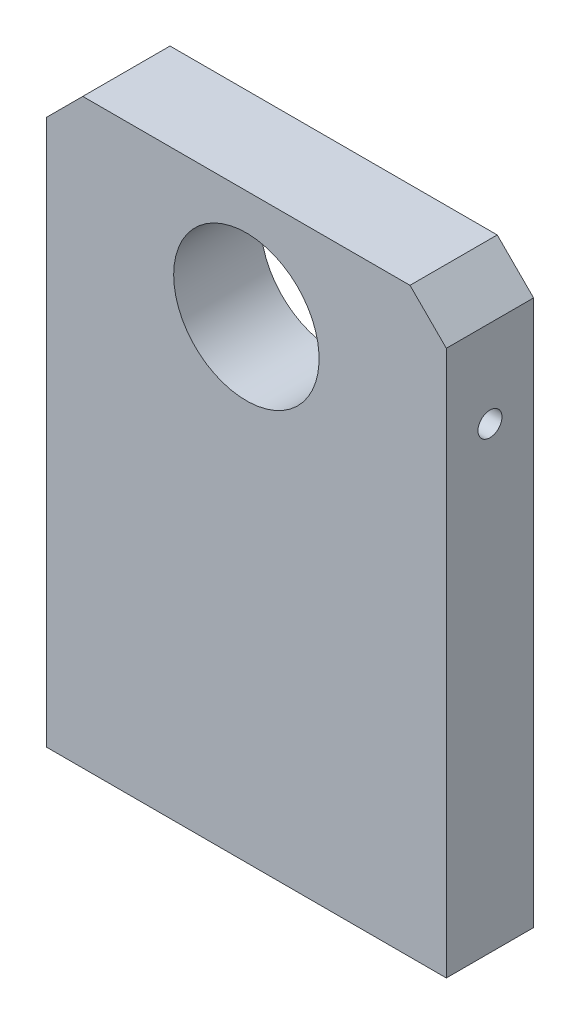
from build123d import *

# Parameters (mm, degrees)
SKETCH_1_W              = 55
SKETCH_1_H              = 80
EXTRUDE_1_DEPTH         = 12
CUT_EXTRUDE_4_REACH     = 52.002
SKETCH_5_R              = 10
CHAMFER_1_SIZE          = 5
HOLE_WIZARD_M4_1_REACH  = 85.845
HOLE_WIZARD_M4_1_BORE_R = 1.65


with BuildPart() as part:
    # 草图1 → 凸台-拉伸1 (new body)
    with BuildSketch(Plane.XY):
        Rectangle(SKETCH_1_W, SKETCH_1_H)
    extrude(amount=EXTRUDE_1_DEPTH)

    # 草图5 → 切除-拉伸4 (cut, up to next)
    with BuildSketch(Plane(origin=(0, 0, 0), x_dir=(-1, 0, 0), z_dir=(0, 0, -1)), mode=Mode.PRIVATE) as cut_extrude_4_sk1:
        with Locations((0, 25)):
            Circle(SKETCH_5_R)
    cut_extrude_4_tool1 = extrude(cut_extrude_4_sk1.sketch, amount=-CUT_EXTRUDE_4_REACH, mode=Mode.PRIVATE) & part.part
    add(cut_extrude_4_tool1.solids().sort_by_distance((0, 25, 0))[0], mode=Mode.SUBTRACT)

    # 倒角1
    chamfer_1_edges = [part.edges().sort_by_distance(p)[0] for p in [
        (-27.5, 40, 6),
        (27.5, 40, 6),
    ]]
    chamfer(chamfer_1_edges, length=CHAMFER_1_SIZE)

    # M4 螺纹孔1 bore (on position points) → M4 螺纹孔1 (cut, up to next)
    with BuildSketch(Plane(origin=(27.5, 23, 6), x_dir=(0, 0, 1), z_dir=(1, 0, 0)), mode=Mode.PRIVATE) as hole_wizard_m4_1_sk1:
        Circle(HOLE_WIZARD_M4_1_BORE_R)
    hole_wizard_m4_1_tool1 = extrude(hole_wizard_m4_1_sk1.sketch, amount=-HOLE_WIZARD_M4_1_REACH, mode=Mode.PRIVATE) & part.part
    add(hole_wizard_m4_1_tool1.solids().sort_by_distance((27.5, 23, 6))[0], mode=Mode.SUBTRACT)


solid = part.part
